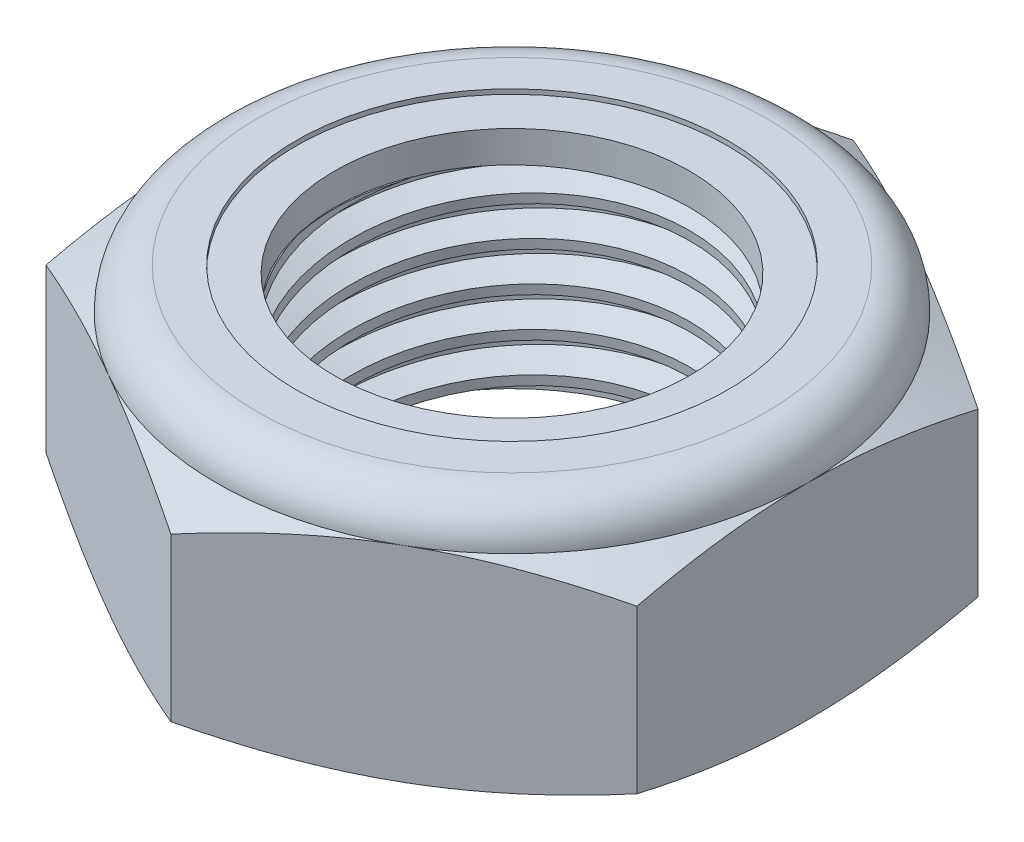
SolidWorks part; units mm, degrees
ref_plane "Front" through (0, 0, 0) normal (0, 0, 1) x (1, 0, 0)
ref_plane "Top" through (0, 0, 0) normal (0, 1, 0) x (1, 0, 0)
ref_plane "Right" through (0, 0, 0) normal (1, 0, 0) x (0, 0, -1)
sketch "Sketch1" plane through (0, 0, 0) normal (0, 1, 0) x (1, 0, 0)
  line L1 (0, 10.9985) -> (-9.525, 5.4993)
  line L2 (-9.525, 5.4993) -> (-9.525, -5.4993)
  line L3 (-9.525, -5.4993) -> (0, -10.9985)
  line L4 (0, -10.9985) -> (9.525, -5.4993)
  line L5 (9.525, -5.4993) -> (9.525, 5.4993)
  line L6 (9.525, 5.4993) -> (0, 10.9985)
  circle A0 centre (0, 0) radius 9.525 construction
  dimension "Hex Flats" = 19.05
extrude "Extrude1" add sketch "Sketch1" along normal blind 7.9375
sketch "Sketch2" plane through (0, 0, 0) normal (1, 0, 0) x (0, 0, -1)
  line L0 (-6.35, 0) -> (-6.35, 7.9375) construction
  line L1 (0, 0) -> (6.35, 0)
  line L2 (0, 0) -> (0, 7.9375)
  line L3 (0, 7.9375) -> (6.35, 7.9375)
  line L4 (6.35, 0) -> (6.35, 7.9375)
  line L5 (-5.4993, 7.9375) -> (5.4993, 7.9375) construction
  line L7 (0, -6.35) -> (0, 0) construction
  dimension "Thread Dia" = 12.7
revolve "Revolve1" add sketch "Sketch2" angle 360 about L7
sketch "Sketch3" plane through (0, 0, 0) normal (1, 0, 0) x (0, 0, -1)
  line L0 (6.35, 7.9375) -> (-6.35, 7.9375) construction
  line L1 (-6.35, 7.9375) -> (-6.35, 6.6675) construction
  line L2 (-6.35, 6.6675) -> (6.35, 7.9375) construction
  line L3 (6.35, 7.9375) -> (6.3658, 7.7795) construction
  line L4 (6.3658, 7.7795) -> (6.4764, 6.6738)
  line L5 (6.4764, 6.6738) -> (5.7529, 7.0003)
  line L6 (5.7529, 7.0003) -> (5.7213, 7.3162)
  line L7 (5.7213, 7.3162) -> (6.3658, 7.7795)
  line L8 (5.7371, 7.1583) -> (6.4211, 7.2267) construction
  line L9 (6.35, 7.9375) -> (6.35, 7.2196) construction
  line L10 (6.35, 7.2196) -> (-6.35, 5.9496) construction
  line L11 (-6.35, 5.9496) -> (-6.35, 6.6675) construction
  line L12 (-0.1353, 7.9375) -> (0.1353, 5.2316) construction
  line L13 (-6.35, 0) -> (-6.35, 7.9375) construction
  line L14 (0, 7.9375) -> (6.35, 7.9375) construction
  line L15 (6.35, 0) -> (6.35, 7.9375) construction
  point P13 (0, 6.5846)
revolve "Cut-Revolve1" cut sketch "Sketch3" angle 360 about L12
pattern_linear "LPattern1" count 6 spacing 1.27 along (0, -1, 0) count 2 spacing 1.27 along (0, 1, 0) seed only of "Cut-Revolve1"
sketch "Sketch4" plane through (0, 0, 0) normal (1, 0, 0) x (0, 0, -1)
  line L0 (0, 7.9375) -> (6.35, 7.9375)
  line L1 (6.35, 7.9375) -> (5.7213, 7.6443)
  line L2 (5.7213, 7.6443) -> (5.7213, 0.2932)
  line L3 (5.7213, 0.2932) -> (6.35, 0)
  line L4 (6.35, 0) -> (0, 0)
  line L5 (0, 0) -> (0, 7.9375)
  line L6 (6.35, 0) -> (6.35, 7.9375) construction
  line L7 (0, 7.9375) -> (6.35, 7.9375) construction
  line L8 (0, 0) -> (6.35, 0) construction
  line L9 (0, 0) -> (0, 7.9375) construction
  line L10 (0, 7.9375) -> (0, 8.6312) construction
  dimension "D1" = 25
revolve "Cut-Revolve2" cut sketch "Sketch4" angle 360 about L10
combine bodies "Combine1" operation type subtract main body 112 bodies to subtract 111
sketch "Sketch5" plane through (0, 0, 0) normal (1, 0, 0) x (0, 0, -1)
  line L0 (0, 0) -> (9.525, 0)
  line L1 (9.525, 0) -> (10.9985, 0.6871)
  line L2 (10.9985, 0.6871) -> (10.9985, 5.9275)
  line L3 (10.9985, 5.9275) -> (9.525, 6.6146)
  line L4 (8.2021, 7.9375) -> (8.2021, 9.2075)
  line L5 (8.2021, 9.2075) -> (12.2685, 9.2075)
  line L6 (12.2685, 9.2075) -> (12.2685, -1.27)
  line L7 (12.2685, -1.27) -> (0, -1.27)
  line L8 (0, -1.27) -> (0, 0)
  line L9 (9.525, 6.6146) -> (9.525, 0) construction
  line L10 (0, 0) -> (6.35, 0) construction
  line L13 (10.9985, 3.3073) -> (12.2685, 3.3073) construction
  line L14 (10.9985, 7.9375) -> (10.9985, 0) construction
  line L15 (0, 0) -> (0, 9.2075) construction
  line L20 (0, 9.2075) -> (8.2021, 9.2075) construction
  line L22 (0, 7.9375) -> (6.35, 7.9375) construction
  arc A0 (9.525, 6.6146) -> (8.2021, 7.9375) centre (8.2021, 6.6146) ccw
revolve "Cut-Revolve3" cut sketch "Sketch5" angle 360 about L15
sketch "Sketch6" plane through (0, 0, 0) normal (1, 0, 0) x (0, 0, -1)
  line L0 (0, 6.6146) -> (9.3726, 6.6146)
  line L1 (8.2021, 7.7851) -> (6.9617, 7.7851)
  line L2 (0, 9.2075) -> (0, 6.6146)
  line L3 (6.9617, 9.2075) -> (0, 9.2075)
  line L4 (0, 9.2075) -> (8.2021, 9.2075) construction
  line L5 (0, 0) -> (0, 9.2075) construction
  line L6 (0, 9.2075) -> (0, 44.323) construction
  line L7 (6.9617, 7.7851) -> (6.9617, 9.2075)
  line L8 (8.2021, 7.9375) -> (8.2021, 7.7851) construction
  line L9 (6.9617, 7.7851) -> (5.7213, 7.7851) construction
  line L10 (5.7213, 7.7851) -> (5.7213, 7.6443) construction
  arc A0 (9.3726, 6.6146) -> (8.2021, 7.7851) centre (8.2021, 6.6146) ccw
  arc A1 (9.525, 6.6146) -> (8.2021, 7.9375) centre (8.2021, 6.6146) ccw construction
  dimension "D1" = 0.1524
revolve "Cut-Revolve4" cut sketch "Sketch6" angle 360 about L6
sketch "Sketch7" plane through (0, 0, 0) normal (1, 0, 0) x (0, 0, -1)
  line L0 (5.7213, 6.6908) -> (9.2937, 6.6908)
  line L1 (8.2021, 7.7089) -> (5.7213, 7.7089)
  line L2 (5.7213, 7.7089) -> (5.7213, 6.6908)
  line L3 (5.7213, 6.6908) -> (0, 6.6908) construction
  line L4 (0, 6.6908) -> (0, 7.7089) construction
  line L5 (0, 7.7089) -> (5.7213, 7.7089) construction
  line L6 (5.7213, 6.6908) -> (5.7213, 6.6146) construction
  line L7 (0, 6.6146) -> (9.3726, 6.6146) construction
  line L8 (8.2021, 7.7089) -> (8.2021, 7.7851) construction
  arc A0 (9.2937, 6.6908) -> (8.2021, 7.7089) centre (8.2021, 6.6146) ccw
  arc A2 (9.3726, 6.6146) -> (8.2021, 7.7851) centre (8.2021, 6.6146) ccw construction
  dimension "D1" = 0.0762
revolve "Revolve2" add sketch "Sketch7" angle 360 about L4
equation "\"D1@Sketch3\"=\"Thread Pitch@Sketch3\"/8"
equation "\"D2@Sketch3\"=\"Thread Pitch@Sketch3\"/4"
equation "\"D5@Sketch3\"=\"Thread Pitch@Sketch3\""
equation "\"D4@LPattern1\"=\"Thread Pitch@Sketch3\""
equation "\"D3@LPattern1\"=\"Thread Pitch@Sketch3\""
equation "\"D1@LPattern1\"=\"Height@Extrude1\"/\"Thread Pitch@Sketch3\""
equation "\"D4@Sketch5\"=\"Height@Extrude1\"/6"
